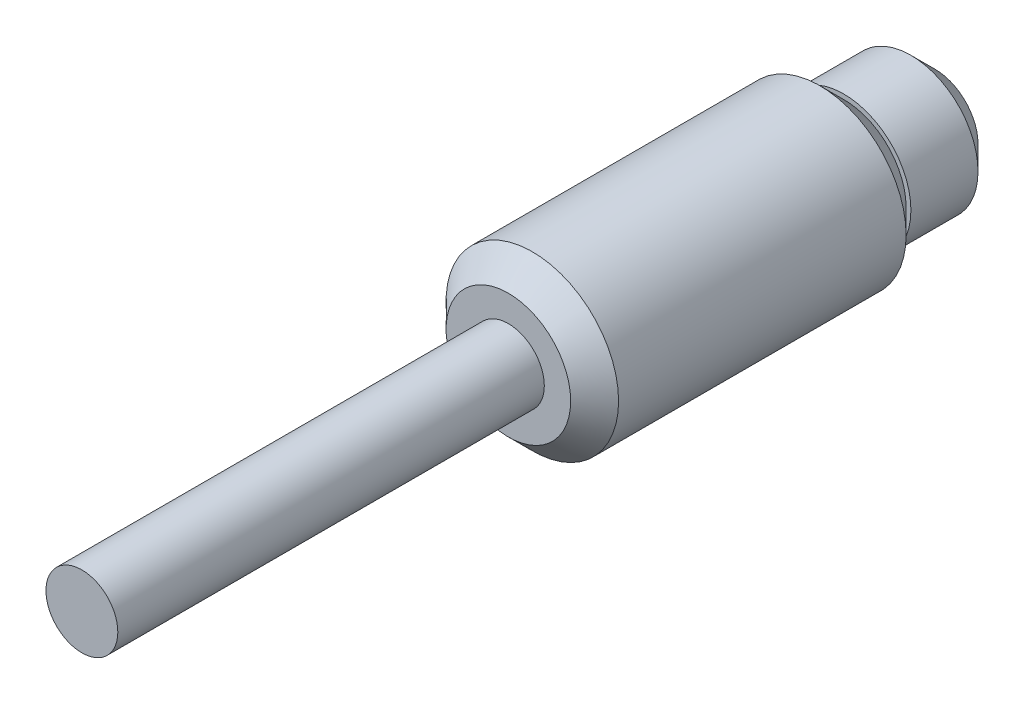
from build123d import *

# Parameters (mm, degrees)
SKETCH_2_R      = 1.8
EXTRUDE_1_DEPTH = 7
SKETCH_3_R      = 0.75
EXTRUDE_2_DEPTH = 8.9
CHAMFER_1_SIZE  = 0.5
CHAMFER_2_SIZE  = 0.5
SKETCH_4_R      = 1.4
EXTRUDE_3_DEPTH = 1.9
CHAMFER_3_SIZE  = 0.5


with BuildPart() as part:
    # 草图2 → 拉伸1 (new body)
    with BuildSketch(Plane.XY):
        Circle(SKETCH_2_R)
    extrude(amount=EXTRUDE_1_DEPTH)

    # 草图3 → 拉伸2 (add)
    with BuildSketch(Plane.XY.offset(7)):
        Circle(SKETCH_3_R)
    extrude(amount=EXTRUDE_2_DEPTH)

    # 倒角1
    chamfer_1_edges = [part.edges().sort_by_distance(p)[0] for p in [
        (-1.8, 0, 0),
    ]]
    chamfer(chamfer_1_edges, length=CHAMFER_1_SIZE)

    # 倒角2
    chamfer_2_edges = [part.edges().sort_by_distance(p)[0] for p in [
        (-1.8, 0, 7),
    ]]
    chamfer(chamfer_2_edges, length=CHAMFER_2_SIZE)

    # 草图4 → 拉伸3 (add)
    with BuildSketch(Plane(origin=(0, 0, 0), x_dir=(-1, 0, 0), z_dir=(0, 0, -1))):
        with Locations(Location((0, 0, 0), (0, 0, 180))):
            Circle(SKETCH_4_R)
    extrude(amount=EXTRUDE_3_DEPTH)

    # 倒角3
    chamfer_3_edges = [part.edges().sort_by_distance(p)[0] for p in [
        (-1.4, 0, -1.9),
    ]]
    chamfer(chamfer_3_edges, length=CHAMFER_3_SIZE)


solid = part.part
